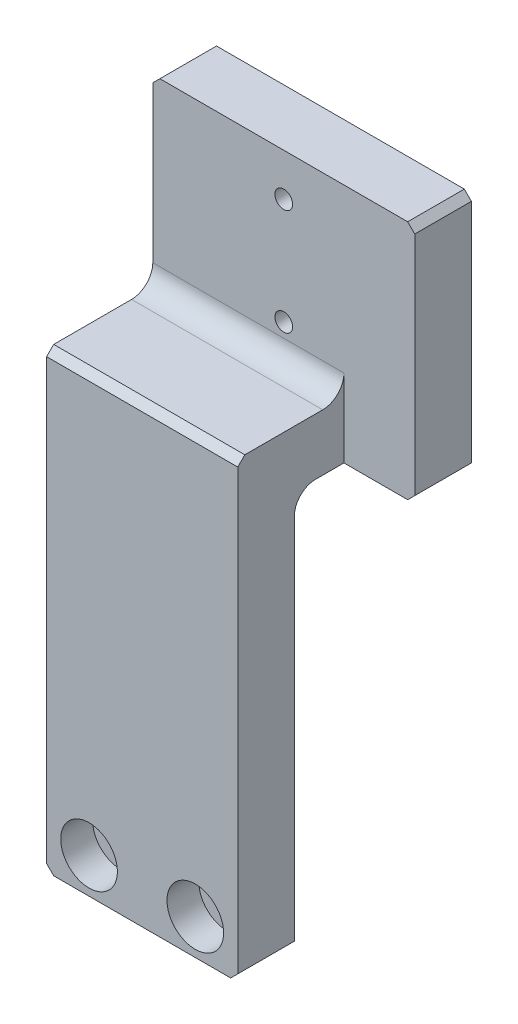
SolidWorks part; units mm, degrees
material "S45C"
ref_plane "Front Plane" through (0, 0, 0) normal (0, 0, 1) x (1, 0, 0)
ref_plane "Top Plane" through (0, 0, 0) normal (0, 1, 0) x (1, 0, 0)
ref_plane "Right Plane" through (0, 0, 0) normal (1, 0, 0) x (0, 0, -1)
sketch "Sketch1" plane through (0, 0, 0) normal (0, 0, 1) x (1, 0, 0)
  line L1 (0, 0) -> (37, 0)
  line L2 (0, 0) -> (0, -90)
  line L3 (0, -90) -> (37, -90)
  line L4 (37, 0) -> (37, -90)
  dimension "D1" = 90
  dimension "D2" = 37
extrude "Boss-Extrude1" add sketch "Sketch1" along normal mid plane 8
sketch "Sketch6" plane through (0, 0, -4) normal (0, 0, 1) x (1, 0, 0)
  line L0 (37, -90) -> (37, 0) construction
  line L1 (0, 0) -> (37, 0)
  line L2 (0, 0) -> (0, -34)
  line L3 (0, -34) -> (37, -34)
  line L4 (37, 0) -> (37, -34)
  dimension "D1" = 34
extrude "Boss-Extrude2" add sketch "Sketch6" against normal blind 15
hole_wizard "M3 Tapped Hole1" positions "Sketch3" profile "Sketch2" tap size "M3" standard "GB" end condition through all
sketch "Sketch3" plane through (0, 0, 4) normal (0, 0, 1) x (1, 0, 0)
  line L1 (37, 0) -> (0, 0) construction
  line L4 (0, 0) -> (0, -90) construction
  point P0 (18.5, -21)
  point P1 (18.5, -6)
  dimension "D1" = 15
  dimension "D2" = 6
  dimension "D3" = 18.5
cosmetic thread "Cosmetic Thread 1" parameters "D2"=3
cosmetic thread "Cosmetic Thread 2" parameters "D2"=3
sketch "Sketch2" plane through (18.5, -21, 4) normal (1, 0, 0) x (0, -1, 0)
  line L0 (0, 0) -> (0, 23)
  line L1 (0, 23) -> (1.25, 23)
  line L2 (1.25, 23) -> (1.25, 0)
  line L5 (1.25, 0) -> (0, 0)
  line L11 (0, -6.35) -> (0, 107.95) construction
  dimension "通孔螺纹孔钻头直径" = 2.5
  dimension "通孔螺纹孔钻头深度" = 23
hole_wizard "CBORE for M4 Hex Head Bolt1" positions "Sketch5" profile "Sketch4" counterbore size "M4" standard "GB" end condition through all
sketch "Sketch5" plane through (0, 0, 4) normal (0, 0, 1) x (1, 0, 0)
  line L0 (0, 0) -> (0, -90) construction
  circle A0 centre (18.5, -21) radius 1.25 construction
  point P0 (6, -85)
  point P2 (21, -85)
  dimension "D1" = 15
  dimension "D2" = 6
  dimension "D3" = 64
sketch "Sketch4" plane through (6, -85, 4) normal (1, 0, 0) x (0, -1, 0)
  line L0 (0, 0) -> (0, 23)
  line L1 (0, 23) -> (2.25, 23)
  line L3 (2.25, 23) -> (2.25, 4.5)
  line L4 (2.25, 4.5) -> (4, 4.5)
  line L5 (4, 4.5) -> (4, 0)
  line L7 (4, 0) -> (0, 0)
  line L11 (0, -6.35) -> (0, 107.95) construction
  dimension "通孔孔直径" = 4.5
  dimension "通孔孔深度" = 23
  dimension "柱形沉头孔直径" = 8
  dimension "柱形沉头孔深度" = 4.5
sketch "Sketch7" plane through (37, 0, 0) normal (1, 0, 0) x (0, 0, -1)
  line L0 (19, -34) -> (19, 0) construction
  line L1 (-4, 0) -> (11, 0)
  line L2 (-4, 0) -> (-4, -26)
  line L3 (-4, -26) -> (11, -26)
  line L4 (11, 0) -> (11, -26)
  line L5 (19, -34) -> (4, -34) construction
  dimension "D1" = 8
  dimension "D2" = 8
extrude "Cut-Extrude1" cut sketch "Sketch7" against normal through all
sketch "Sketch8" plane through (0, 0, 4) normal (0, 0, 1) x (1, 0, 0)
  line L0 (0, -26) -> (37, -26) construction
  line L1 (37, -90) -> (27, -90)
  line L2 (37, -90) -> (37, -26)
  line L3 (37, -26) -> (27, -26)
  line L4 (27, -90) -> (27, -26)
  dimension "D1" = 10
extrude "Cut-Extrude2" cut sketch "Sketch8" against normal up to surface (15 mm away) up to face at (18.5, -4.75, -11)
fillet "Fillet1" radius 3 2 edges at (13.5, -26, -11)
chamfer "Chamfer1" distance 1 angle 45 5 edges at (0, -90, 0) (27, -90, 0) (37, 0, -15) (0, 0, -15)
chamfer "Chamfer2" distance 1 angle 45 2 edges at (13.5, -26, 4) (18, -34, -19)
